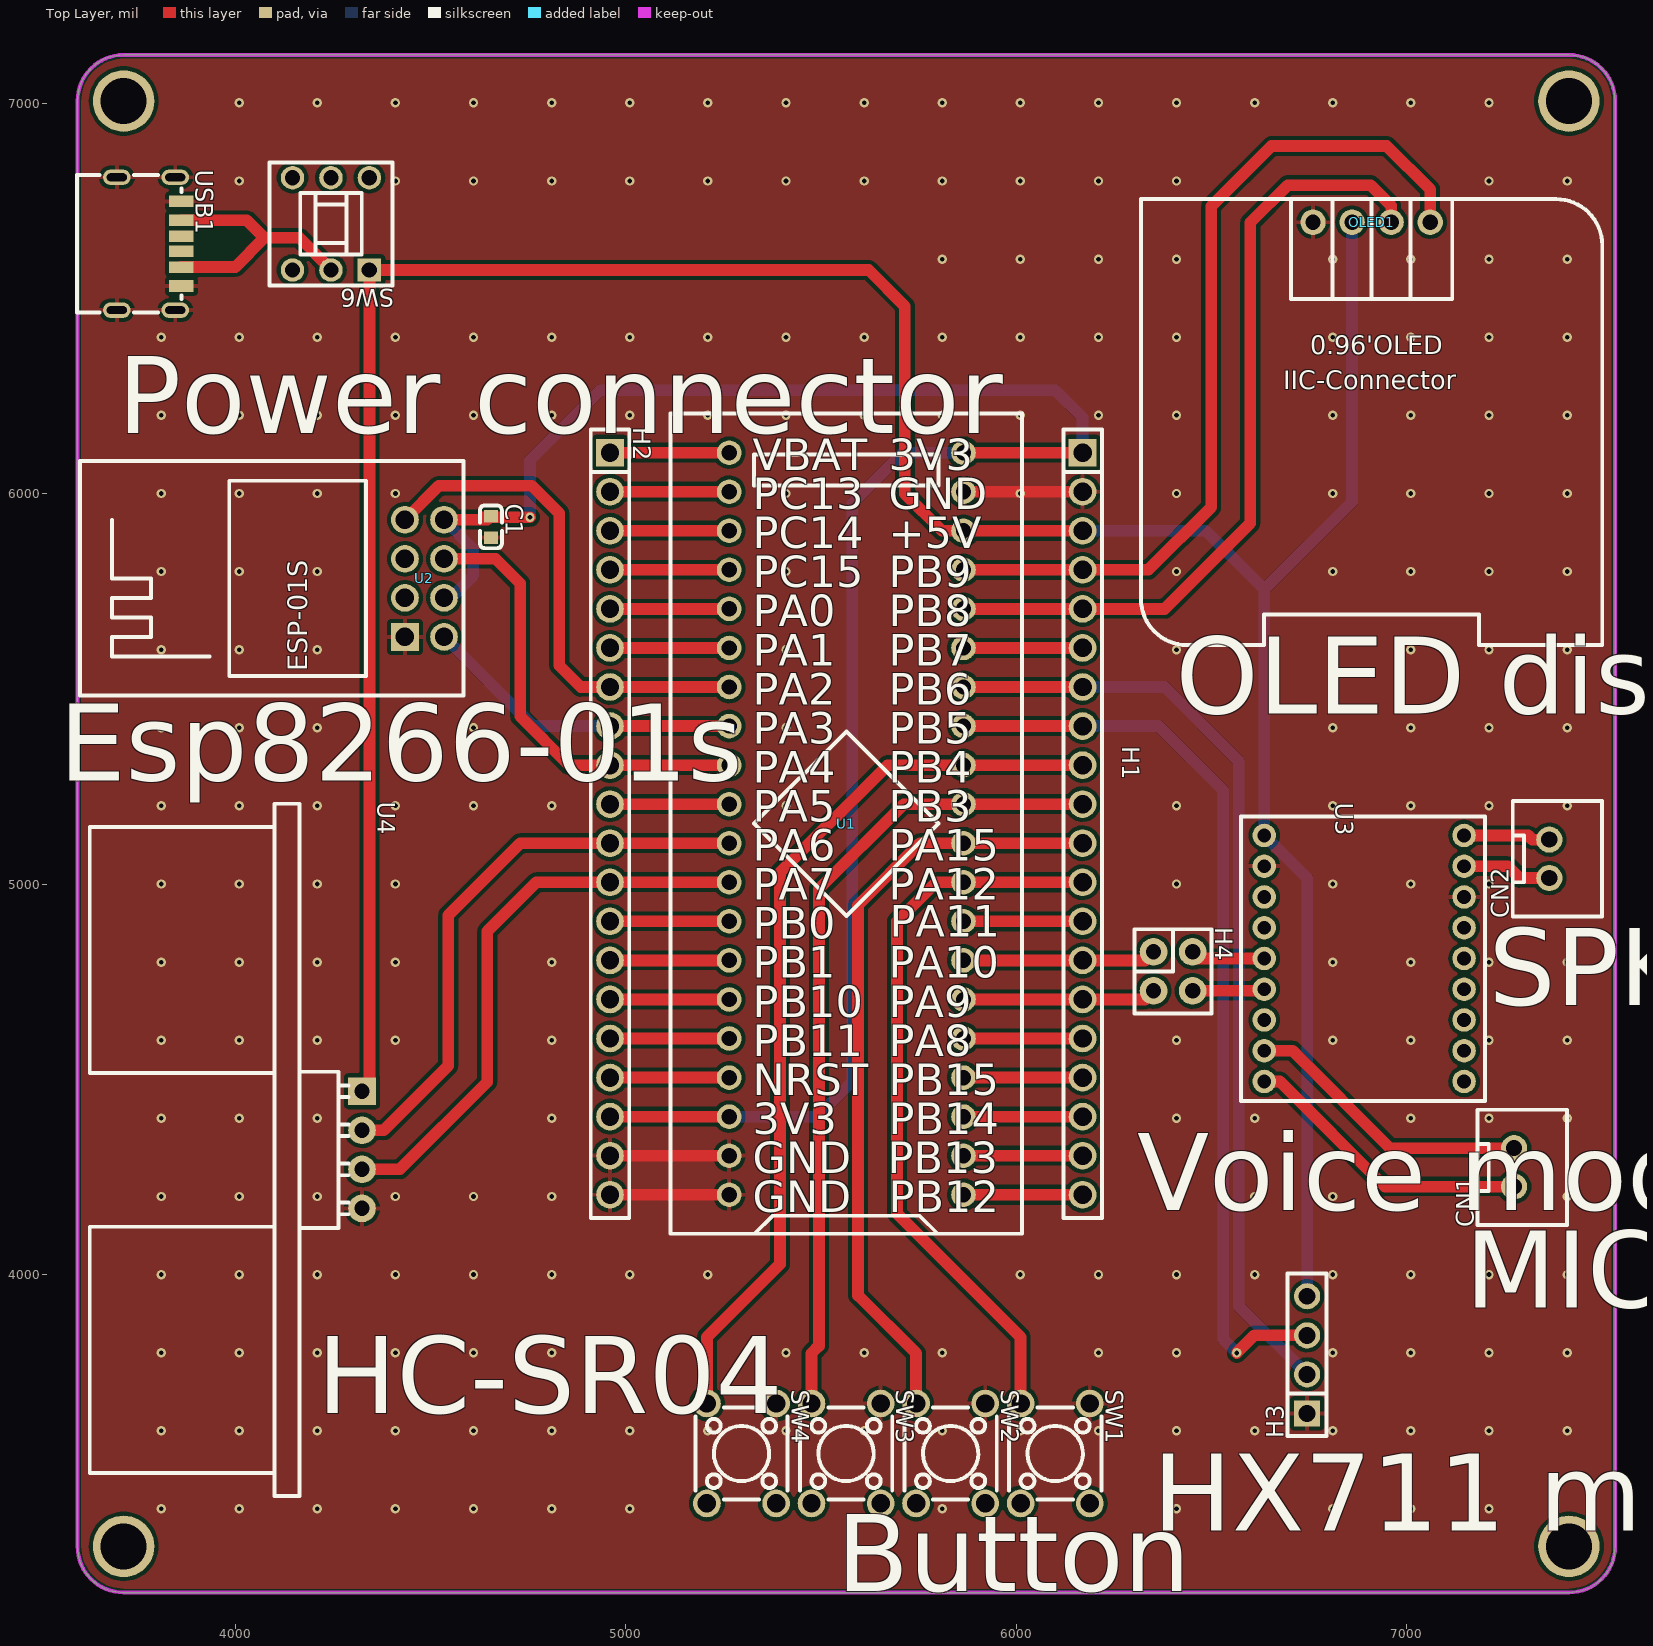
[diagram p0: Top Layer view]
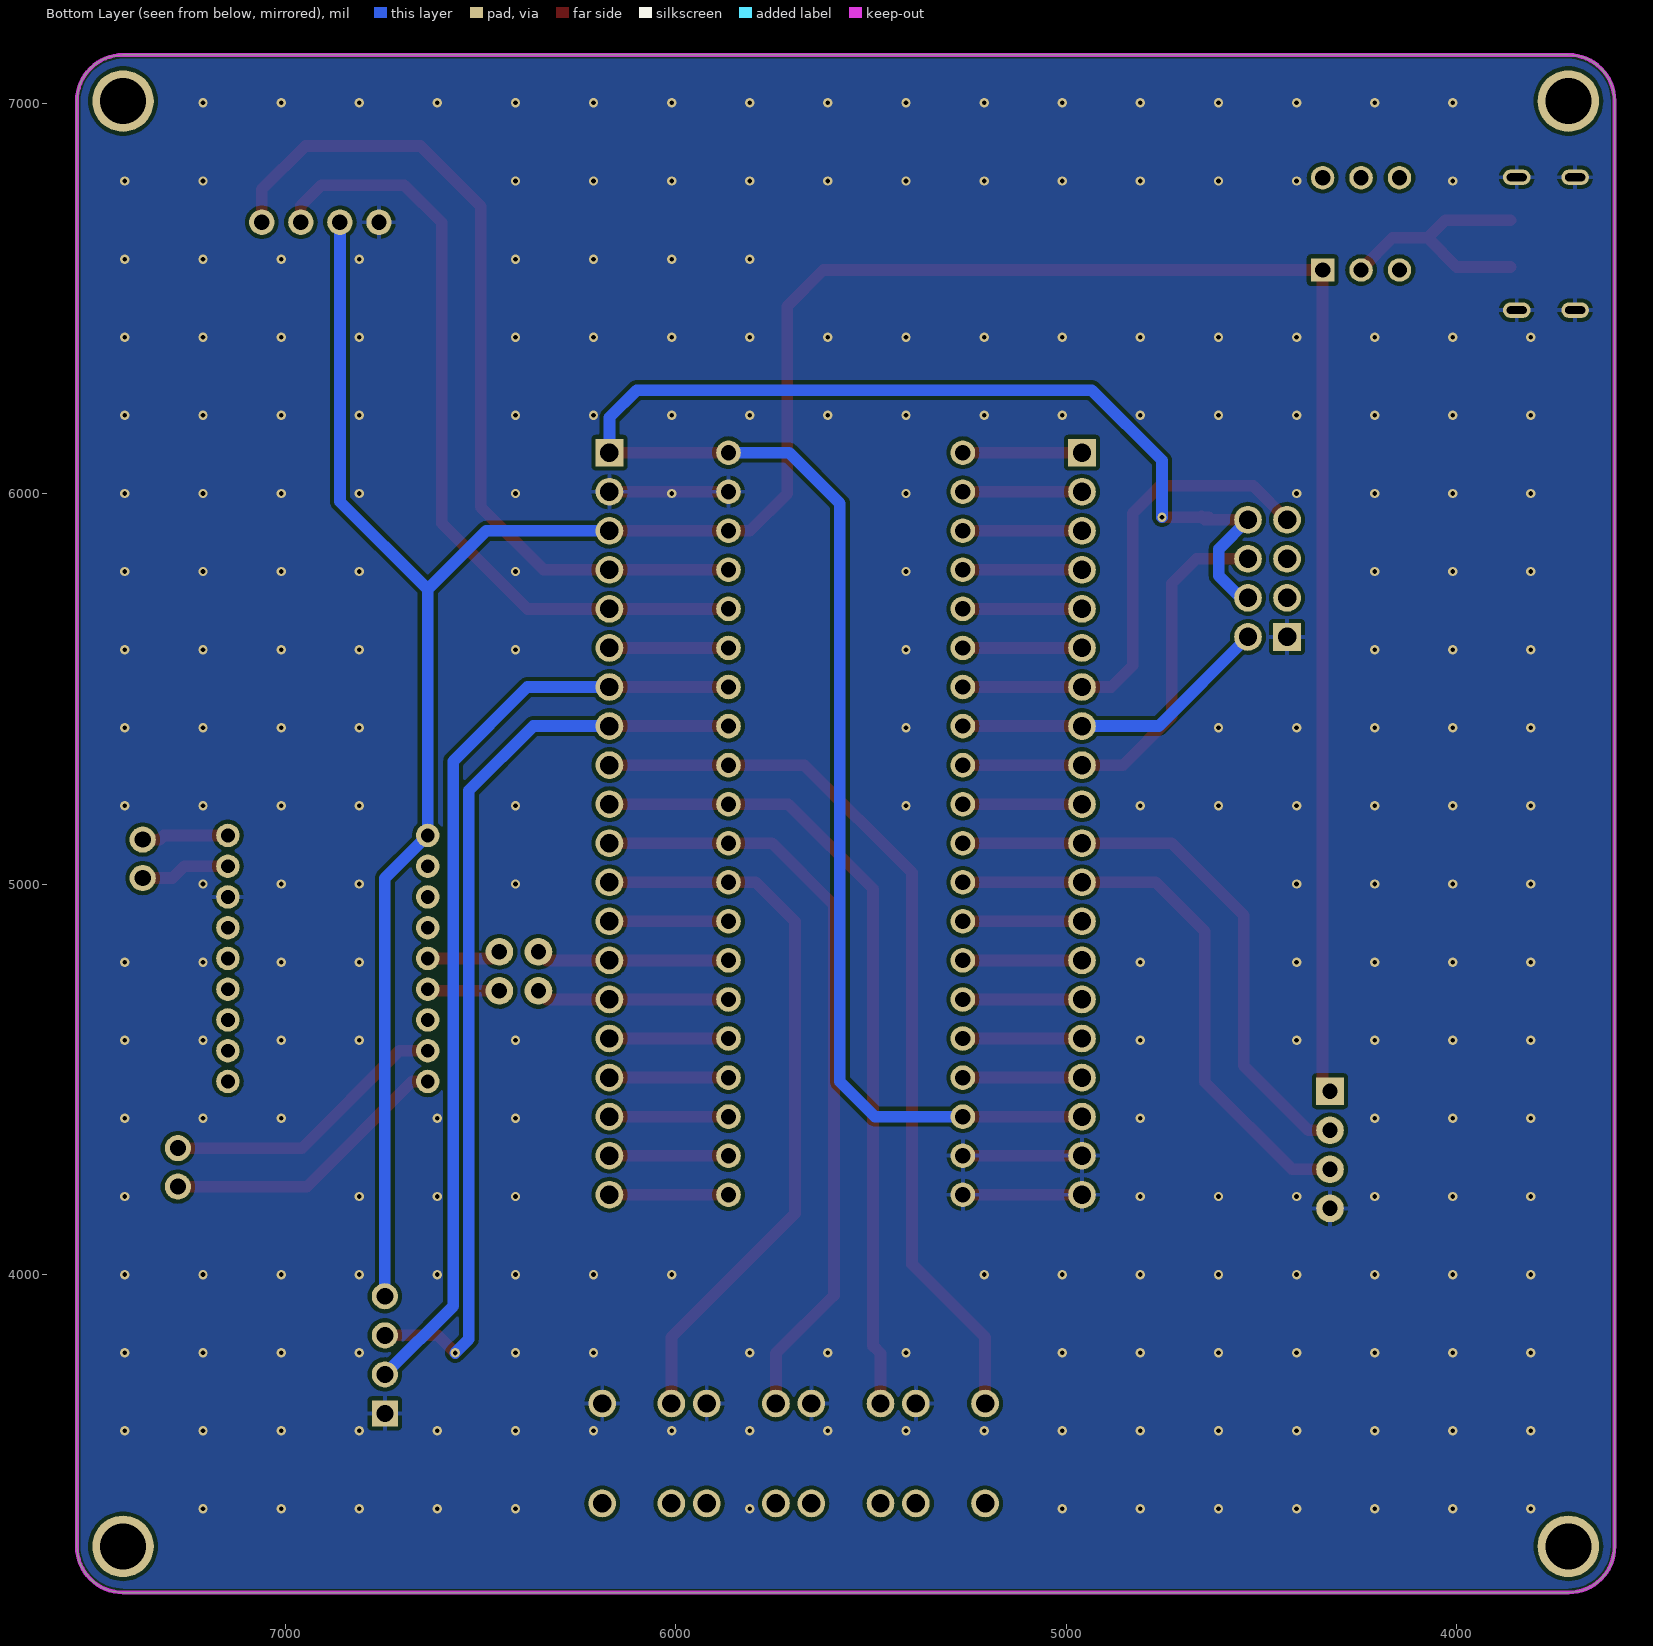
[diagram p1: Bottom Layer view, seen from below]
# Altium PCB MISC89113.pcbdoc
Units mil, origin at the board's own origin, x right, y up, seen from the top; angles counter-clockwise.
Board outline 3937.01 x 3937.01 mil, 2 copper layers (Top Layer, Bottom Layer), stack 62.206 mil thick; 18 components, 46 nets, 164 pads, 238 vias.

## Layer stack, top to bottom
Top Solder Mask Layer: solder mask 0.394, Dk 3.3
Top Layer: signal copper 1.379
Dielectric1: surface 59.449, FR4, Dk 4.5
Bottom Layer: signal copper 1.378
Bottom Solder Mask Layer: solder mask 0.394, Dk 3.3

## Board outline
3714.61,7123.5 ccw(c3714.61,7005.39) 3596.5,7005.39 3596.5,3304.61 ccw(c3714.61,3304.61) 3714.61,3186.5 7415.39,3186.5 ccw(c7415.39,3304.61) 7533.5,3304.61 7533.5,7005.39 ccw(c7415.39,7005.39) 7415.39,7123.5 3714.61,7123.5

## Design rules (kind name [scope] priority, off if disabled: settings)
BoardOutlineClearance copperThickness2oz_1 [All] p2 off: genericclearance=7.99 ignorepadtopadclearanceinfootprint=FALSE except(0: Arc-SplitContinuation Track-SplitContinuation SMDPad-SplitContinuation THPad-SplitContinuation Via-SplitContinuation Fill-SplitContinuation Region-SplitContinuation Poly-SplitContinuation Text-SplitContinuation Hole-SplitContinuation; 5.98: Arc-CutoutEdge Track-CutoutEdge SMDPad-CutoutEdge THPad-CutoutEdge Via-CutoutEdge Text-CutoutEdge; 6.9: Hole-OutlineEdge Hole-CutoutEdge; 10: Poly-OutlineEdge Poly-CutoutEdge; 11.81: Arc-OutlineEdge Track-OutlineEdge SMDPad-OutlineEdge THPad-OutlineEdge Via-OutlineEdge Fill-OutlineEdge Region-OutlineEdge Text-OutlineEdge Fill-CutoutEdge Region-CutoutEdge)
BoardOutlineClearance Plane_innerPlane_1 [All] p4 off: genericclearance=4.02 ignorepadtopadclearanceinfootprint=FALSE except(0: Arc-SplitContinuation Track-SplitContinuation SMDPad-SplitContinuation THPad-SplitContinuation Via-SplitContinuation Fill-SplitContinuation Region-SplitContinuation Poly-SplitContinuation Text-SplitContinuation Hole-SplitContinuation; 5.98: Arc-CutoutEdge Track-CutoutEdge SMDPad-CutoutEdge THPad-CutoutEdge Via-CutoutEdge Text-CutoutEdge; 6.9: Hole-OutlineEdge Hole-CutoutEdge; 10: Poly-OutlineEdge Poly-CutoutEdge; 11.81: Arc-OutlineEdge Track-OutlineEdge SMDPad-OutlineEdge THPad-OutlineEdge Via-OutlineEdge Fill-OutlineEdge Region-OutlineEdge Text-OutlineEdge Fill-CutoutEdge Region-CutoutEdge)
BoardOutlineClearance Copper_copperRegion_1 [All] p6 off: genericclearance=4.02 ignorepadtopadclearanceinfootprint=FALSE except(0: Arc-SplitContinuation Track-SplitContinuation SMDPad-SplitContinuation THPad-SplitContinuation Via-SplitContinuation Fill-SplitContinuation Region-SplitContinuation Poly-SplitContinuation Text-SplitContinuation Hole-SplitContinuation; 5.98: Arc-CutoutEdge Track-CutoutEdge SMDPad-CutoutEdge THPad-CutoutEdge Via-CutoutEdge Text-CutoutEdge; 6.9: Hole-OutlineEdge Hole-CutoutEdge; 10: Poly-OutlineEdge Poly-CutoutEdge; 11.81: Arc-OutlineEdge Track-OutlineEdge SMDPad-OutlineEdge THPad-OutlineEdge Via-OutlineEdge Fill-OutlineEdge Region-OutlineEdge Text-OutlineEdge Fill-CutoutEdge Region-CutoutEdge)
BoardOutlineClearance copperThickness1oz_1 [All] p8: genericclearance=4.02 ignorepadtopadclearanceinfootprint=FALSE except(0: Arc-SplitContinuation Track-SplitContinuation SMDPad-SplitContinuation THPad-SplitContinuation Via-SplitContinuation Fill-SplitContinuation Region-SplitContinuation Poly-SplitContinuation Text-SplitContinuation Hole-SplitContinuation; 5.98: Arc-CutoutEdge Track-CutoutEdge SMDPad-CutoutEdge THPad-CutoutEdge Via-CutoutEdge Text-CutoutEdge; 6.9: Hole-OutlineEdge Hole-CutoutEdge; 10: Poly-OutlineEdge Poly-CutoutEdge; 11.81: Arc-OutlineEdge Track-OutlineEdge SMDPad-OutlineEdge THPad-OutlineEdge Via-OutlineEdge Fill-OutlineEdge Region-OutlineEdge Text-OutlineEdge Fill-CutoutEdge Region-CutoutEdge)
Clearance copperThickness2oz [All] p1 off: gap=7.99 ignorepadtopadclearanceinfootprint=FALSE except(5.98: SMDPad-Track SMDPad-SMDPad THPad-Track SMDPad-THPad THPad-THPad Track-Via SMDPad-Via THPad-Via Via-Via Fill-SMDPad Region-SMDPad Fill-THPad Region-THPad Fill-Via Region-Via Fill-Fill Fill-Region Region-Region Arc-Track Arc-SMDPad Arc-THPad Arc-Via Fill-Arc Region-Arc Arc-Arc Text-Track SMDPad-Text Text-THPad Text-Via Fill-Text Region-Text Arc-Text Text-Text; 6.9: Hole-Track Hole-SMDPad Hole-THPad Hole-Via Fill-Hole Region-Hole Hole-Arc Hole-Text; 10: Poly-Track Poly-SMDPad Poly-THPad Poly-Via Poly-Fill Poly-Region Poly-Poly Poly-Arc Poly-Text Poly-Hole; 11.81: Fill-Track Region-Track)
Clearance Plane_innerPlane [All] p3 off: gap=4.02 ignorepadtopadclearanceinfootprint=FALSE except(5.98: SMDPad-Track SMDPad-SMDPad THPad-Track SMDPad-THPad THPad-THPad Track-Via SMDPad-Via THPad-Via Via-Via Fill-SMDPad Region-SMDPad Fill-THPad Region-THPad Fill-Via Region-Via Fill-Fill Fill-Region Region-Region Arc-Track Arc-SMDPad Arc-THPad Arc-Via Fill-Arc Region-Arc Arc-Arc Text-Track SMDPad-Text Text-THPad Text-Via Fill-Text Region-Text Arc-Text Text-Text; 6.9: Hole-Track Hole-SMDPad Hole-THPad Hole-Via Fill-Hole Region-Hole Hole-Arc Hole-Text; 10: Poly-Track Poly-SMDPad Poly-THPad Poly-Via Poly-Fill Poly-Region Poly-Poly Poly-Arc Poly-Text Poly-Hole; 11.81: Fill-Track Region-Track)
Clearance Copper_copperRegion [All] p5 off: gap=4.02 ignorepadtopadclearanceinfootprint=FALSE except(5.98: SMDPad-Track SMDPad-SMDPad THPad-Track SMDPad-THPad THPad-THPad Track-Via SMDPad-Via THPad-Via Via-Via Fill-SMDPad Region-SMDPad Fill-THPad Region-THPad Fill-Via Region-Via Fill-Fill Fill-Region Region-Region Arc-Track Arc-SMDPad Arc-THPad Arc-Via Fill-Arc Region-Arc Arc-Arc Text-Track SMDPad-Text Text-THPad Text-Via Fill-Text Region-Text Arc-Text Text-Text; 6.9: Hole-Track Hole-SMDPad Hole-THPad Hole-Via Fill-Hole Region-Hole Hole-Arc Hole-Text; 10: Poly-Track Poly-SMDPad Poly-THPad Poly-Via Poly-Fill Poly-Region Poly-Poly Poly-Arc Poly-Text Poly-Hole; 11.81: Fill-Track Region-Track)
Clearance copperThickness1oz [All] p7: gap=4.02 ignorepadtopadclearanceinfootprint=FALSE except(5.98: SMDPad-Track SMDPad-SMDPad THPad-Track SMDPad-THPad THPad-THPad Track-Via SMDPad-Via THPad-Via Via-Via Fill-SMDPad Region-SMDPad Fill-THPad Region-THPad Fill-Via Region-Via Fill-Fill Fill-Region Region-Region Arc-Track Arc-SMDPad Arc-THPad Arc-Via Fill-Arc Region-Arc Arc-Arc Text-Track SMDPad-Text Text-THPad Text-Via Fill-Text Region-Text Arc-Text Text-Text; 6.9: Hole-Track Hole-SMDPad Hole-THPad Hole-Via Fill-Hole Region-Hole Hole-Arc Hole-Text; 10: Poly-Track Poly-SMDPad Poly-THPad Poly-Via Poly-Fill Poly-Region Poly-Poly Poly-Arc Poly-Text Poly-Hole; 11.81: Fill-Track Region-Track)
DiffPairsRouting differentialPair [All] p1: maxlimit=6 minlimit=6 mostfreqgap=6 toplayer_minwidth=5 toplayer_prefwidth=10 toplayer_maxwidth=100 toplayer_mingap=6 toplayer_prefgap=6 toplayer_maxgap=6 bottomlayer_minwidth=5 bottomlayer_prefwidth=10 bottomlayer_maxwidth=100 bottomlayer_mingap=6 bottomlayer_prefgap=6 bottomlayer_maxgap=6 maxuncoupledlength=10
HoleToHoleClearance otherClearance [All] p1: gap=11.81 allowstackedmicrovias=TRUE
Length netLength [All] p1: minlimit=0 maxlimit=0
PasteMaskExpansion pasteMaskExpansion [All] p1: expansion=0
PlaneConnect innerPlane [All] p1: planeconnectstyle=Relief reliefexpansion=20 reliefentries=4 reliefconductorwidth=10 reliefairgap=10
PolygonConnect copperRegion [All] p1: connectstyle=Relief reliefconductorwidth=10 reliefentries=4 polygonreliefangle="90 Angle" airgapwidth=10 via.connectstyle=Relief via.reliefconductorwidth=10 via.reliefentries=4 via.polygonreliefangle="90 Angle" via.airgapwidth=10
RoutingVias viaSize [All] p1: holewidth=12.01 width=24.02 viastyle="Through Hole" minholewidth=11.81 minwidth=19.68 maxholewidth=248.03 maxwidth=393.7
SolderMaskExpansion solderMaskExpansion [IsVia] p1: expansion=-1000 istentingtop=TRUE
SolderMaskExpansion solderMaskExpansion [All] p2: expansion=2 istentingtop=FALSE
Width copperThickness2oz_2 [All] p1 off: maxlimit=100 minlimit=8 preferedwidth=10
Width copperThickness1oz_2 [All] p2: maxlimit=100 minlimit=5 preferedwidth=10

## Components (designator, comment, footprint, x,y, rotation, side; value= is the part's Value field where it differs from the comment)
C1 "100nF" C0603 4655,5915 r270 top
CN1 "XH2.54*2P_Through-hole" CONN-TH_2P-P2.50-XH2.54-2P 7275,4275 r90 top
CN2 "XH2.54*2P_Through-hole" CONN-TH_2P-P2.50-XH2.54-2P 7365,5065 r90 top
H1 "" HDR-TH_20P-P2.54-V-F 6170,5155 r270 top
H2 "" HDR-TH_20P-P2.54-V-F 4960,5155 r270 top
H3 "" HDR-TH_4P-P2.54-V-F 6745,3795 r90 top
H4 "" HDR-TH_4P-P2.54-V-F-R2-C2-S2.54 6401.72,4776.97 r270 top
OLED1 "" 0.96OLED_4P 6910,6695 r0 top
SW1 "" SW-TH_4P-L6.0-W6.0-P4.50-LS6.5 6099.85,3542.47 r270 top
SW2 "" SW-TH_4P-L6.0-W6.0-P4.50-LS6.5 5832.14,3542.47 r270 top
SW3 "" SW-TH_4P-L6.0-W6.0-P4.50-LS6.5 5564.43,3542.47 r270 top
SW4 "" SW-TH_4P-L6.0-W6.0-P4.50-LS6.5 5296.72,3542.47 r270 top
SW6 "PS081-06L135D1-JF-G" SW-TH_6P-L8.0-W8.0-P2.50-TL 4245.52,6690.75 r180 top
U1 "STM32F103C8T6-Card" CONN-TH_L53.3-W22.9_STM32F103C8T6-CARD 5565,5155 r90 top
U2 "ESP-01S" WIFIM-TH_ESP-01S 4485,5783.21 r90 top
U3 "CON2.0MM-PAD-18" CONN-TH_18P-P2.00_C9900078766 6635,4810 r270 top
U4 "HC-SR04" TH_HC-SR04V 4325,4320 r270 top
USB1 "TYPEC-250D-BCP6" USB-C-SMD_TYPEC-250D-BCP6 3780,6640 r270 top

## Footprints (in the part's own frame and the unit in brackets; to place one, negate y for a bottom-side part, rotate by r counter-clockwise, add the part's x,y. Pads: shape width x height; smd on the part's side, far side on the other; paste and mask are expansions set on the pad)
0.96OLED_4P [mm]
  round 1.65 hole 1 copper offset 0,0: 1(-3.81,-0.001) 2(-1.27,0.002) 3(1.27,0.002) 4(3.81,0.002)
  silkscreen extent -15,-27.5 15,1.5
C0603 [mm]
  rect 0.8x0.9 smd: 1(-0.7,0) 2(0.7,0)
  silkscreen extent -1.39,-0.71 1.39,0.71
CONN-TH_2P-P2.50-XH2.54-2P [mm]
  round 1.7 hole 1.05 paste+0 mask+0.05: 1(1.25,0) 2(-1.25,0)
  silkscreen extent -3.75,-3.42 3.75,2.37
CONN-TH_18P-P2.00_C9900078766 [mil]
  round 60 hole 35.43 paste+0 mask+1.97: 1(-314.96,0.01) 2(-314.96,511.81) 3(-236.22,0.01) 4(-236.22,511.81) 5(-157.48,0.01) 6(-157.48,511.81) 9(0,0) 10(0,511.81) 11(78.74,0) 12(78.74,511.81) 13(157.48,0) 14(157.48,511.81) 15(236.22,0) 16(236.22,511.81) 17(314.96,0) 18(314.96,511.81)
  round 60 hole 35.43 copper offset -0.01,0 paste+0 mask+1.97: 7(-78.72,0.01) 8(-78.72,511.81)
  silkscreen extent -363,-60 365,565
CONN-TH_L53.3-W22.9_STM32F103C8T6-CARD [mm]
  round 1.6 hole 1: 1(-24.13,-7.62) 2(-21.59,-7.62) 3(-19.05,-7.62) 4(-16.51,-7.62) 5(-13.97,-7.62) 6(-11.43,-7.62) 7(-8.89,-7.62) 8(-6.35,-7.62) 9(-3.81,-7.62) 10(-1.27,-7.62) 11(1.27,-7.62) 12(3.81,-7.62) 13(6.35,-7.62) 14(8.89,-7.62) 15(11.43,-7.62) 16(13.97,-7.62) 17(16.51,-7.62) 18(19.05,-7.62) 19(21.59,-7.62) 20(24.13,-7.62) 21(24.13,7.62) 22(21.59,7.62) 23(19.05,7.62) 24(16.51,7.62) 25(13.97,7.62) 26(11.43,7.62) 27(8.89,7.62) 28(6.35,7.62) 29(3.81,7.62) 30(1.27,7.62) 31(-1.27,7.62) 32(-3.81,7.62) 33(-6.35,7.62) 34(-8.89,7.62) 35(-11.43,7.62) 36(-13.97,7.62) 37(-16.51,7.62) 38(-19.05,7.62) 39(-21.59,7.62) 40(-24.13,7.62)
  silkscreen extent -26.67,-11.43 26.67,11.43
HDR-TH_4P-P2.54-V-F [mm]
  rect 1.7x1.7 hole 1.1: 1(-3.81,0)
  round 1.7 hole 1.1: 2(-1.27,0) 3(1.27,0) 4(3.81,0)
  silkscreen extent -5.29,-1.27 5.29,1.27
HDR-TH_4P-P2.54-V-F-R2-C2-S2.54 [mm]
  round 1.8 hole 1: 1(-1.27,-1.27) 2(-1.27,1.27) 3(1.27,-1.27) 4(1.27,1.27)
  silkscreen extent -2.74,-2.5 2.74,2.5
HDR-TH_20P-P2.54-V-F [mm]
  rect 1.8x1.8 hole 1.2: 1(-24.13,0)
  round 1.8 hole 1.2: 2(-21.59,0) 3(-19.05,0) 4(-16.51,0) 5(-13.97,0) 6(-11.43,0) 7(-8.89,0) 8(-6.35,0) 9(-3.81,0) 10(-1.27,0) 11(1.27,0) 12(3.81,0) 13(6.35,0) 14(8.89,0) 15(11.43,0) 16(13.97,0) 17(16.51,0) 18(19.05,0) 19(21.59,0) 20(24.13,0)
  silkscreen extent -25.65,-1.25 25.65,1.25
SW-TH_4P-L6.0-W6.0-P4.50-LS6.5 [mm]
  round 1.8 hole 1.2: 1(-3.25,2.25) 2(3.25,2.25) 3(-3.25,-2.25) 4(3.25,-2.25)
  silkscreen extent -3,-3 3,3
SW-TH_6P-L8.0-W8.0-P2.50-TL [mil]
  rect 60x60 hole 39.37: 1(-98.43,118.11)
  round 60 hole 39.37: 2(0,118.11) 3(98.42,118.11) 4(-98.43,-118.11) 5(0,-118.11) 6(98.42,-118.11)
  silkscreen extent -157,-157 157,157
TH_HC-SR04V [mm]
  rect 1.8x1.8 hole 1.001: 1(-3.81,0)
  round 1.8 hole 1.001: 2(-1.27,0) 3(1.27,0) 4(3.81,0)
  silkscreen extent -22.5,-17.7 22.5,-0.89
USB-C-SMD_TYPEC-250D-BCP6 [mm]
  oval 1x1.8 hole 0.5 slot 1.3 at 90 deg paste+0 mask+0.05: 1(-4.32,1.7) 2(-4.32,-2.1) 3(4.32,-2.1) 4(4.32,1.7)
  rect 0.75x1.6 smd paste-100 mask+0.05: A5(-0.5,2.1) A9(1.52,2.1) B5(0.5,2.1) B9(-1.52,2.1)
  rect 0.75x1.6 smd paste-100 mask+0.051: A12(2.75,2.1) B12(-2.75,2.1)
  silkscreen extent -4.48,-4.7 4.47,2.1
WIFIM-TH_ESP-01S [mm]
  rect 1.8x1.8 hole 1.2: 1(-3.81,1.27)
  round 1.8 hole 1.2: 2(-1.27,1.27) 3(1.27,1.27) 4(3.81,1.27) 5(3.81,-1.27) 6(1.27,-1.27) 7(-1.27,-1.27) 8(-3.81,-1.27)
  silkscreen extent -7.62,-2.54 7.62,22.4

## Free pads (board coordinates)
  round 157.48 hole 118.11: 1(3714.61,7005.39) 1(3714.61,3304.61) 1(7415.39,7005.39) 1(7415.39,3304.61)

## Via types
v1: diameter 24.02, hole 12, Top Layer to Bottom Layer, 238 vias

## Nets (pads, with @x,y where several pads share a name; then routed paths per layer and width w, separated by ;. In a path a pad name is that pad's centre, name@x,y a point inside that pad or via, vN(x,y) a via of type N, cw(c..) or ccw(c..) an arc to the next point about the centre after c; other vN are vias at no path point)
$1N17258: H4.2 U3.9 | length 190.3
  Top Layer w30: H4.2 6468.69,4810 U3.9
$1N17259: H4.4 U3.11 | length 185.1
  Top Layer w30: H4.4 6630.71,4726.97 U3.11
+3V3: C1.1 H1.1 H2.18 U1.20 U1.38 U2.5 U2.7 | length 5056.4
  Top Layer w30: U2.5 4645.65,5933.21 C1.1@4652.44,5940 ; 4635,5940 C1.1@4652.44,5940 ; C1.1 C1.1@4652.44,5940 ; v1(4755,5940) C1.1@4652.44,5940 ; H2.18@4955,4405 U1.38 ; U1.20 H1.1
  Bottom Layer w30: U2.7 4553.21,5733.21 4610,5790 4610,5858.21 U2.5 ; v1(4755,5940) 4755,6085 4935,6265 6100,6265 6170,6195 H1.1 ; U1.38 5490,4405 5580,4495 5580,5975 5710,6105 U1.20
+5V: H1.3 H3.4 OLED1.2 SW6.1 U1.18 U3.1 U4.1 | length 7910.2
  Top Layer w30: U4.1 4343.95,4488.95 SW6.1 5622.36,6572.64 5715,6480 5715,6000.09 5810.08,5905 U1.18 H1.3
  Bottom Layer w30: H1.3 6485,5905 6635.01,5754.99 ; H3.4 6745,5014.97 U3.1 6635.01,5754.99 ; OLED1.2@6860,6695.05 6860,5979.98 6635.01,5754.99
GND: C1.2 H1.2 H2.19 H2.20 H3.1 OLED1.1 SW1.1 SW2.1 SW3.1 SW4.1 U1.19 U1.39 U1.40 U2.1 U3.3 U3.6 U4.4 USB1.1 USB1.2 USB1.3 USB1.4 USB1.A12 USB1.B12 | length 925
  Top Layer w30: H2.20@4955,4205 U1.40 ; H2.19@4955,4305 U1.39 ; U1.19 H1.2
  other v1: 3810.6,3400.6 4010.6,3400.6 4210.6,3400.6 4410.6,3400.6 4610.6,3400.6 4810.6,3400.6 5010.6,3400.6 5810.6,3400.6 6410.6,3400.6 6610.6,3400.6 6810.6,3400.6 7010.6,3400.6 7210.6,3400.6 3810.6,3600.6 4010.6,3600.6 4210.6,3600.6 4410.6,3600.6 4610.6,3600.6 4810.6,3600.6 5010.6,3600.6 5210.6,3600.6 5410.6,3600.6 5610.6,3600.6 5810.6,3600.6 6010.6,3600.6 6210.6,3600.6 6410.6,3600.6 6610.6,3600.6 6810.6,3600.6 7010.6,3600.6 7210.6,3600.6 7410.6,3600.6 3810.6,3800.6 4010.6,3800.6 4210.6,3800.6 4410.6,3800.6 4610.6,3800.6 4810.6,3800.6 5010.6,3800.6 5410.6,3800.6 5610.6,3800.6 5810.6,3800.6 6210.6,3800.6 6410.6,3800.6 6810.6,3800.6 7010.6,3800.6 7210.6,3800.6 7410.6,3800.6 3810.6,4000.6 4010.6,4000.6 4210.6,4000.6 4410.6,4000.6 4610.6,4000.6 4810.6,4000.6 5010.6,4000.6 5210.6,4000.6 6010.6,4000.6 6210.6,4000.6 6410.6,4000.6 6610.6,4000.6 6810.6,4000.6 7010.6,4000.6 7210.6,4000.6 7410.6,4000.6 3810.6,4200.6 4010.6,4200.6 4210.6,4200.6 4410.6,4200.6 4610.6,4200.6 4810.6,4200.6 6410.6,4200.6 6610.6,4200.6 6810.6,4200.6 7410.6,4200.6 3810.6,4400.6 4010.6,4400.6 4210.6,4400.6 4810.6,4400.6 6410.6,4400.6 6610.6,4400.6 7010.6,4400.6 7210.6,4400.6 7410.6,4400.6 3810.6,4600.6 4010.6,4600.6 4210.6,4600.6 4410.6,4600.6 4810.6,4600.6 6410.6,4600.6 6810.6,4600.6 7010.6,4600.6 7210.6,4600.6 7410.6,4600.6 3810.6,4800.6 4010.6,4800.6 4210.6,4800.6 4410.6,4800.6 4810.6,4800.6 6810.6,4800.6 7010.6,4800.6 7210.6,4800.6 7410.6,4800.6 3810.6,5000.6 4010.6,5000.6 4210.6,5000.6 4410.6,5000.6 6410.6,5000.6 6810.6,5000.6 7010.6,5000.6 7210.6,5000.6 3810.6,5200.6 4010.6,5200.6 4210.6,5200.6 4410.6,5200.6 4610.6,5200.6 4810.6,5200.6 5410.6,5200.6 6410.6,5200.6 6810.6,5200.6 7010.6,5200.6 7210.6,5200.6 7410.6,5200.6 3810.6,5400.6 4010.6,5400.6 4210.6,5400.6 4410.6,5400.6 4610.6,5400.6 5410.6,5400.6 6810.6,5400.6 7010.6,5400.6 7210.6,5400.6 7410.6,5400.6 3810.6,5600.6 4010.6,5600.6 4210.6,5600.6 5410.6,5600.6 6410.6,5600.6 6810.6,5600.6 7010.6,5600.6 7210.6,5600.6 7410.6,5600.6 3810.6,5800.6 4010.6,5800.6 4210.6,5800.6 5410.6,5800.6 6410.6,5800.6 6810.6,5800.6 7010.6,5800.6 7210.6,5800.6 7410.6,5800.6 3810.6,6000.6 4010.6,6000.6 4210.6,6000.6 4410.6,6000.6 5410.6,6000.6 6010.6,6000.6 6410.6,6000.6 6810.6,6000.6 7010.6,6000.6 7210.6,6000.6 7410.6,6000.6 3810.6,6200.6 4010.6,6200.6 4210.6,6200.6 4410.6,6200.6 4610.6,6200.6 4810.6,6200.6 5010.6,6200.6 5210.6,6200.6 5410.6,6200.6 5610.6,6200.6 5810.6,6200.6 6010.6,6200.6 6210.6,6200.6 6410.6,6200.6 6810.6,6200.6 7010.6,6200.6 7210.6,6200.6 7410.6,6200.6 3810.6,6400.6 4010.6,6400.6 4210.6,6400.6 4410.6,6400.6 4610.6,6400.6 4810.6,6400.6 5010.6,6400.6 5210.6,6400.6 5410.6,6400.6 5610.6,6400.6 5810.6,6400.6 6010.6,6400.6 6210.6,6400.6 6410.6,6400.6 6810.6,6400.6 7010.6,6400.6 7210.6,6400.6 7410.6,6400.6 5810.6,6600.6 6010.6,6600.6 6210.6,6600.6 6410.6,6600.6 6810.6,6600.6 7010.6,6600.6 7210.6,6600.6 7410.6,6600.6 4010.6,6800.6 4410.6,6800.6 4610.6,6800.6 4810.6,6800.6 5010.6,6800.6 5210.6,6800.6 5410.6,6800.6 5610.6,6800.6 5810.6,6800.6 6010.6,6800.6 6210.6,6800.6 6410.6,6800.6 7210.6,6800.6 7410.6,6800.6 4010.6,7000.6 4210.6,7000.6 4410.6,7000.6 4610.6,7000.6 4810.6,7000.6 5010.6,7000.6 5210.6,7000.6 5410.6,7000.6 5610.6,7000.6 5810.6,7000.6 6010.6,7000.6 6210.6,7000.6 6410.6,7000.6 6610.6,7000.6 6810.6,7000.6 7010.6,7000.6 7210.6,7000.6
MIC+: CN1.1 U3.15 | length 743.4
  Top Layer w30: U3.15 6707.62,4573.78 6957.18,4324.22 CN1.1
MIC-: CN1.2 U3.17 | length 751.5
  Top Layer w30: U3.17 6675,4495.04 6944.26,4225.78 CN1.2
PA0: H2.5 U1.25 | length 310
  Top Layer w30: H2.5@4955,5705 U1.25
PA1: H2.6 U1.26 | length 310
  Top Layer w30: H2.6@4955,5605 U1.26
PA2_TX_WIFI: H2.7 U1.27 U2.4 | length 1307.7
  Top Layer w30: U2.4 4521.79,6020 4760,6020 4830,5950 4830,5560 4885,5505 H2.7 U1.27
PA3_RX_WIFI: H2.8 U1.28 U2.8 | length 829.5
  Top Layer w30: H2.8@4955,5405 U1.28
  Bottom Layer w30: U2.8 4763.21,5405 H2.8
PA4_WIFIRST: H2.9 U1.29 U2.6 | length 1148
  Top Layer w30: U2.6 4666.79,5833.21 4730,5770 4730,5430 4855,5305 H2.9 U1.29
PA5: H2.10 U1.30 | length 310
  Top Layer w30: H2.10@4955,5205 U1.30
PA6_TRIG: H2.11 U1.31 U4.2 | length 1470.4
  Top Layer w30: U4.2 4380.71,4370 4545.71,4535 4545.71,4920.71 4730,5105 U1.31
PA7_ECHO: H2.12 U1.32 U4.3 | length 1470.4
  Top Layer w30: U4.3 4422.13,4270 4645.71,4493.58 4645.71,4879.29 4771.42,5005 U1.32
PA8: H1.16 U1.5 | length 305
  Top Layer w30: U1.5 H1.16
PA9: U3.8
PA9_TX_SU03T: H1.15 H4.3 U1.6 | length 495.8
  Top Layer w30: U1.6 H1.15 6329.74,4705 H4.3
PA10: U3.10
PA10_RX_SU03T: H1.14 H4.1 U1.7 | length 495.8
  Top Layer w30: U1.7 H1.14 6329.74,4805 H4.1
PA11: H1.13 U1.8 | length 305
  Top Layer w30: U1.8 H1.13
PA12_KEY1: H1.12 SW1.3 U1.9 | length 1882
  Top Layer w30: SW1.3 6011.27,3840.12 5695,4156.39 5695,4905 5795,5005 U1.9 H1.12
PA15_KEY2: H1.11 SW2.3 U1.10 | length 1978.2
  Top Layer w30: SW2.3 5743.56,3798.7 5595,3947.25 5595,4946.42 5753.58,5105 U1.10 H1.11
PB0: H2.13 U1.33 | length 310
  Top Layer w30: H2.13@4955,4905 U1.33
PB1: H2.14 U1.34 | length 310
  Top Layer w30: H2.14@4955,4805 U1.34
PB3_KEY3: H1.10 SW3.3 U1.11 | length 2090.3
  Top Layer w30: SW3.3 5475.85,3798.7 5495,3817.85 5495,4987.84 5712.16,5205 U1.11 H1.10
PB4_KEY4: H1.9 SW4.3 U1.12 | length 2325.5
  Top Layer w30: SW4.3 5208.14,3840.12 5395,4026.98 5395,5029.26 5670.74,5305 U1.12 H1.9
PB5_SCK: H1.8 H3.3 U1.13 | length 2386.5
  Top Layer w30: U1.13 H1.8 ; v1(6565,3800) 6610,3845 H3.3
  Bottom Layer w30: H1.8 6365,5405 6530,5240 6530,3835 v1(6565,3800)
PB6_SDA: H1.7 H3.2 U1.14 | length 2426.2
  Top Layer w30: U1.14 H1.7
  Bottom Layer w30: H1.7 6380,5505 6570,5315 6570,3920 H3.2
PB7: H1.6 U1.15 | length 305
  Top Layer w30: U1.15 H1.6
PB8_OLEDSCL: H1.5 OLED1.3 U1.16 | length 2059.7
  Top Layer w30: U1.16 H1.5 6380,5705 6599.29,5924.29 6599.29,6694.29 6695,6790 6907.53,6790 6960,6737.53 OLED1.3@6960,6695.05
PB9_OLEDSDA: H1.4 OLED1.4 U1.17 | length 2225.4
  Top Layer w30: U1.17 H1.4 6338.58,5805 6499.29,5965.71 6499.29,6735.71 6653.58,6890 6948.95,6890 7060,6778.95 OLED1.4@7060,6695.05
PB10: H2.15 U1.35 | length 310
  Top Layer w30: H2.15@4955,4705 U1.35
PB11: H2.16 U1.36 | length 310
  Top Layer w30: H2.16@4955,4605 U1.36
PB12: H1.20 U1.1 | length 305
  Top Layer w30: U1.1 H1.20
PB13: H1.19 U1.2 | length 305
  Top Layer w30: U1.2 H1.19
PB14: H1.18 U1.3 | length 305
  Top Layer w30: U1.3 H1.18
PB15: H1.17 U1.4 | length 305
  Top Layer w30: U1.4 H1.17
PC13_BEEP: H2.2 U1.22 | length 310
  Top Layer w30: H2.2@4955,6005 U1.22
PC14: H2.3 U1.23 | length 310
  Top Layer w30: H2.3@4955,5905 U1.23
PC15: H2.4 U1.24 | length 310
  Top Layer w30: H2.4@4955,5805 U1.24
RST: H2.17 U1.37 | length 310
  Top Layer w30: H2.17@4955,4505 U1.37
SPK+: CN2.1 U3.2 | length 222.6
  Top Layer w30: U3.2 7310.79,5124.96 7321.54,5114.22 CN2.1
SPK-: CN2.2 U3.4 | length 230.8
  Top Layer w30: U3.4 7258.49,5046.22 7288.92,5015.78 CN2.2
VBAT: H2.1 U1.21 | length 310
  Top Layer w30: H2.1@4955,6105 U1.21
VBUS: SW6.2 USB1.A9 USB1.B9 | length 679.9
  Top Layer w30: USB1.A9 4000.16,6580.16 4075,6655 ; USB1.B9 4030.15,6699.85 4075,6655 ; SW6.2 4245.52,6574.48 4165,6655 4075,6655
pads on no net: SW1.2 SW1.4 SW2.2 SW2.4 SW3.2 SW3.4 SW4.2 SW4.4 SW6.3 SW6.4 SW6.5 SW6.6 U2.2 U2.3 U3.5 U3.7 U3.12 U3.13 U3.14 U3.16 U3.18 USB1.A5 USB1.B5

## Polygon pours and split planes (outlines as drawn)
GND on Bottom Layer (solid, remove dead copper, pour order 2): 3525,7245 3525,3080 7700,3080 7700,7245
GND on Top Layer (solid, remove dead copper, pour order 2): 3000,7415 3000,3000 7930,3000 7930,7415

## Keep-outs
Board Outline Layer:
  the board outline again, w10

## Silkscreen, mask and mechanical layers (free items; w line width, h text height)
Top Silkscreen Layer:
  text "Power connector" at 3700,6155 h196.85
  text "VBAT" at 5325.95,6060 h80
  text "3V3" at 5674.16,6060 h80
  text "PC13" at 5325.95,5960 h80
  text "GND" at 5674.16,5960 h80
  text "PC14" at 5325.95,5860 h80
  text "+5V" at 5674.16,5860 h80
  text "PC15" at 5325.95,5760 h80
  text "PB9" at 5674.16,5760 h80
  text "PA0" at 5325.95,5660 h80
  text "PB8" at 5674.16,5660 h80
  text "PA1" at 5325.95,5560 h80
  text "PB7" at 5674.16,5560 h80
  text "PA2" at 5325.95,5460 h80
  text "PB6" at 5674.16,5460 h80
  text "OLED display" at 6408.66,5436.57 h196.85
  text "PA3" at 5325.95,5360 h80
  text "PB5" at 5674.16,5360 h80
  text "Esp8266-01s" at 3550,5265 h196.85
  text "PA4" at 5325.95,5260 h80
  text "PB4" at 5674.16,5260 h80
  text "PA5" at 5325.95,5160 h80
  text "PB3" at 5674.16,5160 h80
  text "PA6" at 5325.95,5060 h80
  text "PA15" at 5674.16,5060 h80
  text "PA7" at 5325.95,4960 h80
  text "PA12" at 5674.16,4960 h80
  text "PA11" at 5675.95,4865 h80
  text "PB0" at 5325.95,4860 h80
  text "PB1" at 5325.95,4760 h80
  text "PA10" at 5674.16,4760 h80
  text "SPK" at 7210,4690 h196.85
  text "PB10" at 5325.95,4660 h80
  text "PA9" at 5674.16,4660 h80
  text "PB11" at 5325.95,4560 h80
  text "PA8" at 5674.16,4560 h80
  text "NRST" at 5325.95,4460 h80
  text "PB15" at 5674.16,4460 h80
  text "3V3" at 5325.95,4360 h80
  text "PB14" at 5674.16,4360 h80
  text "GND" at 5325.95,4260 h80
  text "PB13" at 5670.95,4260 h80
  text "Voice module" at 6310,4165 h196.85
  text "GND" at 5325.95,4160 h80
  text "PB12" at 5674.16,4160 h80
  text "MIC" at 7150,3915 h196.85
  text "HC-SR04" at 4210,3645 h196.85
  text "HX711 module" at 6350,3345 h196.85
  text "Button" at 5540,3190 h196.85